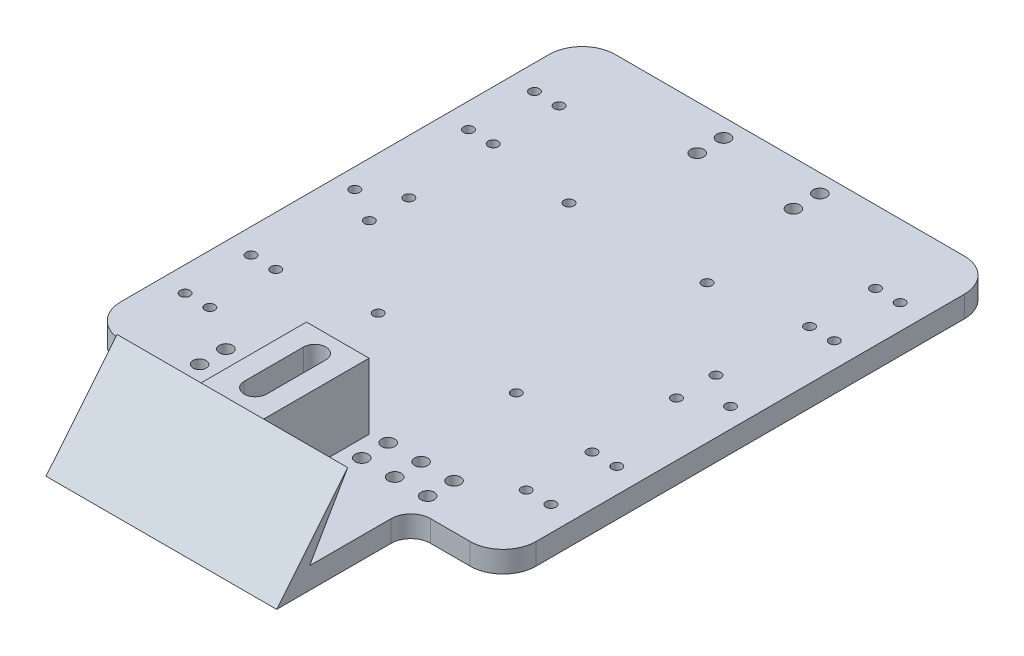
SolidWorks part; units mm, degrees
ref_plane "Front Plane" through (0, 0, 0) normal (0, 0, 1) x (1, 0, 0)
ref_plane "Top Plane" through (0, 0, 0) normal (0, 1, 0) x (1, 0, 0)
ref_plane "Right Plane" through (0, 0, 0) normal (1, 0, 0) x (0, 0, -1)
other "Configuration Table"
sketch "Sketch1" plane through (0, 0, 0) normal (0, 1, 0) x (1, 0, 0)
  line L1 (-63, -75) -> (63, -75)
  line L2 (-63, -75) -> (-63, 75)
  line L3 (-63, 75) -> (63, 75)
  line L4 (63, -75) -> (63, 75)
  line L5 (0, 75) -> (0, -75) construction
  line L6 (-63, 0) -> (63, 0) construction
  point P0 (0, 0)
  dimension "D1" = 126
  dimension "D2" = 150
extrude "Boss-Extrude1" add sketch "Sketch1" along normal blind 6.5
sketch "Sketch2" plane through (0, 6.5, 0) normal (0, 1, 0) x (1, 0, 0)
  line L0 (63, 75) -> (-63, 75) construction
  line L1 (-55.5, 33) -> (-48, 33) construction
  line L2 (-55.5, 33) -> (-55.5, 53) construction
  line L3 (-55.5, 53) -> (-48, 53) construction
  line L4 (-48, 33) -> (-48, 53) construction
  line L5 (-51.75, 53) -> (-51.75, 33) construction
  line L6 (-55.5, 43) -> (-48, 43) construction
  line L7 (-63, 75) -> (-63, -75) construction
  circle A0 centre (-55.5, 33) radius 1.5
  circle A1 centre (-48, 33) radius 1.5
  circle A2 centre (-48, 53) radius 1.5
  circle A3 centre (-55.5, 53) radius 1.5
  point P0 (-51.75, 43)
  dimension "D3" = 3
  dimension "D1" = 20
  dimension "D2" = 7.5
  dimension "D4" = 22
  dimension "D5" = 7.5
extrude "Cut-Extrude1" cut sketch "Sketch2" against normal blind 10
mirror "Mirror1" about plane through (0, 0, 0) normal (1, 0, 0) of "Cut-Extrude1"
mirror "Mirror2" about plane through (0, 0, 0) normal (0, 0, 1) of "Cut-Extrude1", "Mirror1"
sketch "Sketch3" plane through (0, 6.5, 0) normal (0, 1, 0) x (1, 0, 0)
  line L1 (-20.95, -28.95) -> (20.95, -28.95) construction
  line L2 (-20.95, -28.95) -> (-20.95, 28.95) construction
  line L3 (-20.95, 28.95) -> (20.95, 28.95) construction
  line L4 (20.95, -28.95) -> (20.95, 28.95) construction
  line L5 (0, 28.95) -> (0, -28.95) construction
  line L6 (-20.95, 0) -> (20.95, 0) construction
  circle A0 centre (-20.95, -28.95) radius 1.5
  circle A1 centre (20.95, -28.95) radius 1.5
  circle A2 centre (20.95, 28.95) radius 1.5
  circle A3 centre (-20.95, 28.95) radius 1.5
  point P0 (0, 0)
  dimension "D3" = 3
  dimension "D1" = 41.9
  dimension "D2" = 57.9
extrude "Cut-Extrude2" cut sketch "Sketch3" against normal blind 10
fillet "Fillet1" radius 10 4 edges at (63, 3.25, 75) (-63, 3.25, 75) (63, 3.25, -75) (-63, 3.25, -75)
sketch "Sketch4" plane through (0, 6.5, 0) normal (0, 1, 0) x (1, 0, 0)
  line L0 (-63, 65) -> (-63, -65) construction
  line L1 (-57, 0) -> (-46.6077, -6) construction
  line L2 (-46.6077, -6) -> (-46.6077, 6) construction
  line L3 (-46.6077, 6) -> (-57, 0) construction
  circle A0 centre (-50.0718, 0) radius 3.4641 construction
  circle A1 centre (-46.6077, -6) radius 1.5
  circle A2 centre (-46.6077, 6) radius 1.5
  circle A3 centre (-57, 0) radius 1.5
  dimension "D3" = 3
  dimension "D1" = 12
  dimension "D2" = 6
extrude "Cut-Extrude3" cut sketch "Sketch4" against normal blind 10
mirror "Mirror3" about plane through (0, 0, 0) normal (1, 0, 0) of "Cut-Extrude3"
sketch "Sketch5" plane through (0, 6.5, 0) normal (0, 1, 0) x (1, 0, 0)
  line L0 (-53, -75) -> (53, -75) construction
  line L1 (63, -65) -> (63, 65) construction
  circle A0 centre (14.61, -61.5) radius 2
  circle A1 centre (14.61, -69.5) radius 2
  dimension "D1" = 4
  dimension "D2" = 13.5
  dimension "D3" = 48.39
  dimension "D4" = 8
extrude "Cut-Extrude4" cut sketch "Sketch5" against normal blind 20
mirror "Mirror4" about plane through (0, 0, 0) normal (1, 0, 0) of "Cut-Extrude4"
mirror "Mirror5" about plane through (0, 0, 0) normal (0, 0, 1) of "Cut-Extrude4", "Mirror4"
sketch "Sketch6" plane through (0, 6.5, 0) normal (0, 1, 0) x (1, 0, 0)
  line L0 (0, -75) -> (0, -58.6445) construction
  line L1 (-53, -75) -> (53, -75) construction
  circle A0 centre (14.61, -69.5) radius 2 construction
  circle A1 centre (14.61, -69.5) radius 2
  circle A2 centre (14.61, -61.5) radius 2 construction
  circle A3 centre (14.61, -61.5) radius 2
  circle A4 centre (24.61, -69.5) radius 2
  circle A5 centre (24.61, -61.5) radius 2
  circle A6 centre (34.61, -69.5) radius 2
  circle A7 centre (34.61, -61.5) radius 2
  circle A8 centre (-34.61, -61.5) radius 2
  circle A9 centre (-34.61, -69.5) radius 2
  circle A10 centre (-24.61, -61.5) radius 2
  circle A11 centre (-24.61, -69.5) radius 2
  circle A12 centre (-14.61, -61.5) radius 2
  circle A13 centre (-14.61, -69.5) radius 2
  dimension "D1" = 10
  dimension "D2" = 3
extrude "Cut-Extrude5" cut sketch "Sketch6" against normal through all
sketch "Sketch8" plane through (0, 0, 0) normal (1, 0, 0) x (0, 0, -1)
  line L0 (-75, 0) -> (-115.71, 0)
  line L1 (-115.71, 0) -> (-94.163, 26.5)
  line L2 (-94.163, 26.5) -> (-105.71, 6.5)
  line L3 (-105.71, 6.5) -> (-75, 6.5)
  line L4 (-75, 0) -> (-75, 6.5) construction
  line L5 (-75, 0) -> (-75, 6.5)
  dimension "D1" = 30.71
  dimension "D2" = 60
  dimension "D3" = 10
  dimension "D4" = 20
extrude "Boss-Extrude3" add sketch "Sketch8" along normal mid plane 70
sketch "Sketch9" plane through (0, 0, 0) normal (1, 0, 0) x (0, 0, -1)
  line L0 (-94.163, 26.5) -> (-62.163, 26.5)
  line L2 (-62.163, 26.5) -> (-62.163, 6.5)
  line L3 (-65, 6.5) -> (65, 6.5) construction
  line L4 (-62.163, 6.5) -> (-75, 6.5)
  line L5 (-75, 0) -> (-75, 6.5)
  line L6 (-75, 6.5) -> (-105.71, 6.5)
  line L7 (-105.71, 6.5) -> (-94.163, 26.5)
  line L8 (-94.163, 26.5) -> (-115.71, 0)
  line L9 (-115.71, 0) -> (-75, 0)
  line L11 (-75, 6.5) -> (-105.71, 6.5)
  line L12 (-105.71, 6.5) -> (-94.163, 26.5)
  dimension "D2" = 32
  dimension "D1" = 0
extrude "Boss-Extrude4" add sketch "Sketch9" along normal mid plane 19
sketch "Sketch10" plane through (0, 26.5, 0) normal (0, 1, 0) x (1, 0, 0)
  line L0 (0, -87.163) -> (0, -69.163) construction
  line L1 (-3.386, -87.163) -> (-3.386, -69.163)
  line L2 (3.386, -87.163) -> (3.386, -69.163)
  line L3 (9.5, -62.163) -> (-9.5, -62.163) construction
  arc A0 (-3.386, -87.163) -> (3.386, -87.163) centre (0, -87.163) ccw
  arc A1 (3.386, -69.163) -> (-3.386, -69.163) centre (0, -69.163) ccw
  point P2 (0, -78.163)
  dimension "D1" = 16
  dimension "D2" = 18
extrude "Cut-Extrude6" cut sketch "Sketch10" against normal through all
fillet "Fillet2" radius 6 2 edges at (-35, 3.25, 75) (35, 3.25, 75)
